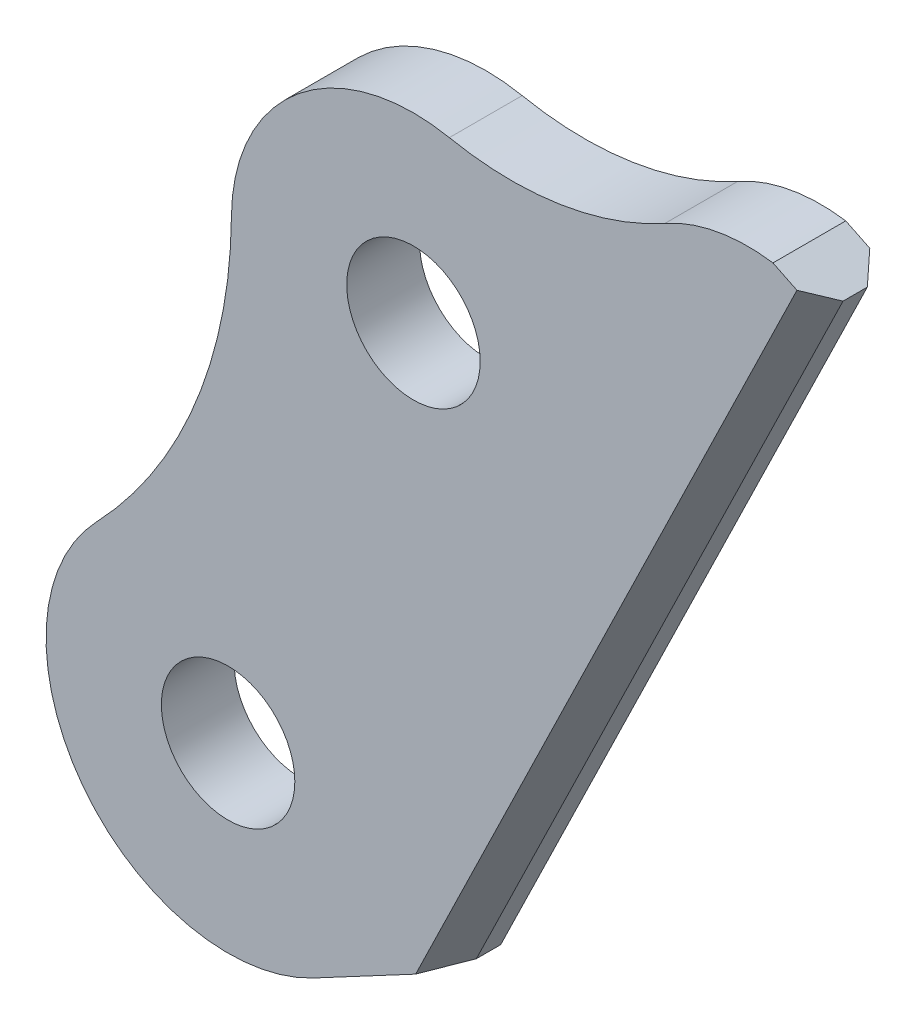
SolidWorks part; units mm, degrees
ref_plane "Front Plane" through (0, 0, 0) normal (0, 0, 1) x (1, 0, 0)
ref_plane "Top Plane" through (0, 0, 0) normal (0, 1, 0) x (1, 0, 0)
ref_plane "Right Plane" through (0, 0, 0) normal (1, 0, 0) x (0, 0, -1)
sketch "Sketch1" plane through (0, 0, 0) normal (0, 0, 1) x (1, 0, 0)
  line L0 (-48.2058, 0) -> (91.432, 0) construction
  line L1 (0, 53.5031) -> (0, -53.0793) construction
  line L2 (0, 0) -> (76.3735, 188.0853) construction
  line L3 (92.3, -35.8) -> (243.3735, 274.3853)
  line L4 (92.3, -35.8) -> (35.27, -66.1893)
  line L5 (243.3735, 274.3853) -> (224.4937, 283.5806)
  arc A0 (-54.1686, 51.8725) -> (35.27, -66.1893) centre (0, 0) ccw
  arc A1 (91.1595, 261.6134) -> (1.3757, 188.6618) centre (76.3735, 188.0853) ccw
  circle A2 centre (76.3735, 188.0853) radius 27.5
  circle A3 centre (0, 0) radius 27.5
  arc A4 (-54.1686, 51.8725) -> (1.3757, 188.6618) centre (-198.6183, 190.1992) ccw
  arc A5 (224.4937, 283.5806) -> (180.0634, 275.5001) centre (214.1344, 214.3514) ccw
  arc A6 (91.1595, 261.6134) -> (180.0634, 275.5001) centre (116.7886, 389.062) ccw
  dimension "D1" = 150
  dimension "D4" = 55
  dimension "D5" = 55
  dimension "D6" = 150
  dimension "D7" = 400
  dimension "D13" = 140
  dimension "D14" = 260
  dimension "D2" = 67.9
  dimension "D3" = 203
  dimension "D8" = 35.8
  dimension "D9" = 92.3
  dimension "D10" = 167
  dimension "D11" = 86.3
  dimension "D12" = 21
extrude "Boss-Extrude1" add sketch "Sketch1" along normal blind 30
chamfer "Chamfer1" distance 10 angle 45 2 edges at (167.8368, 119.2927, 0) (167.8368, 119.2927, 30)
